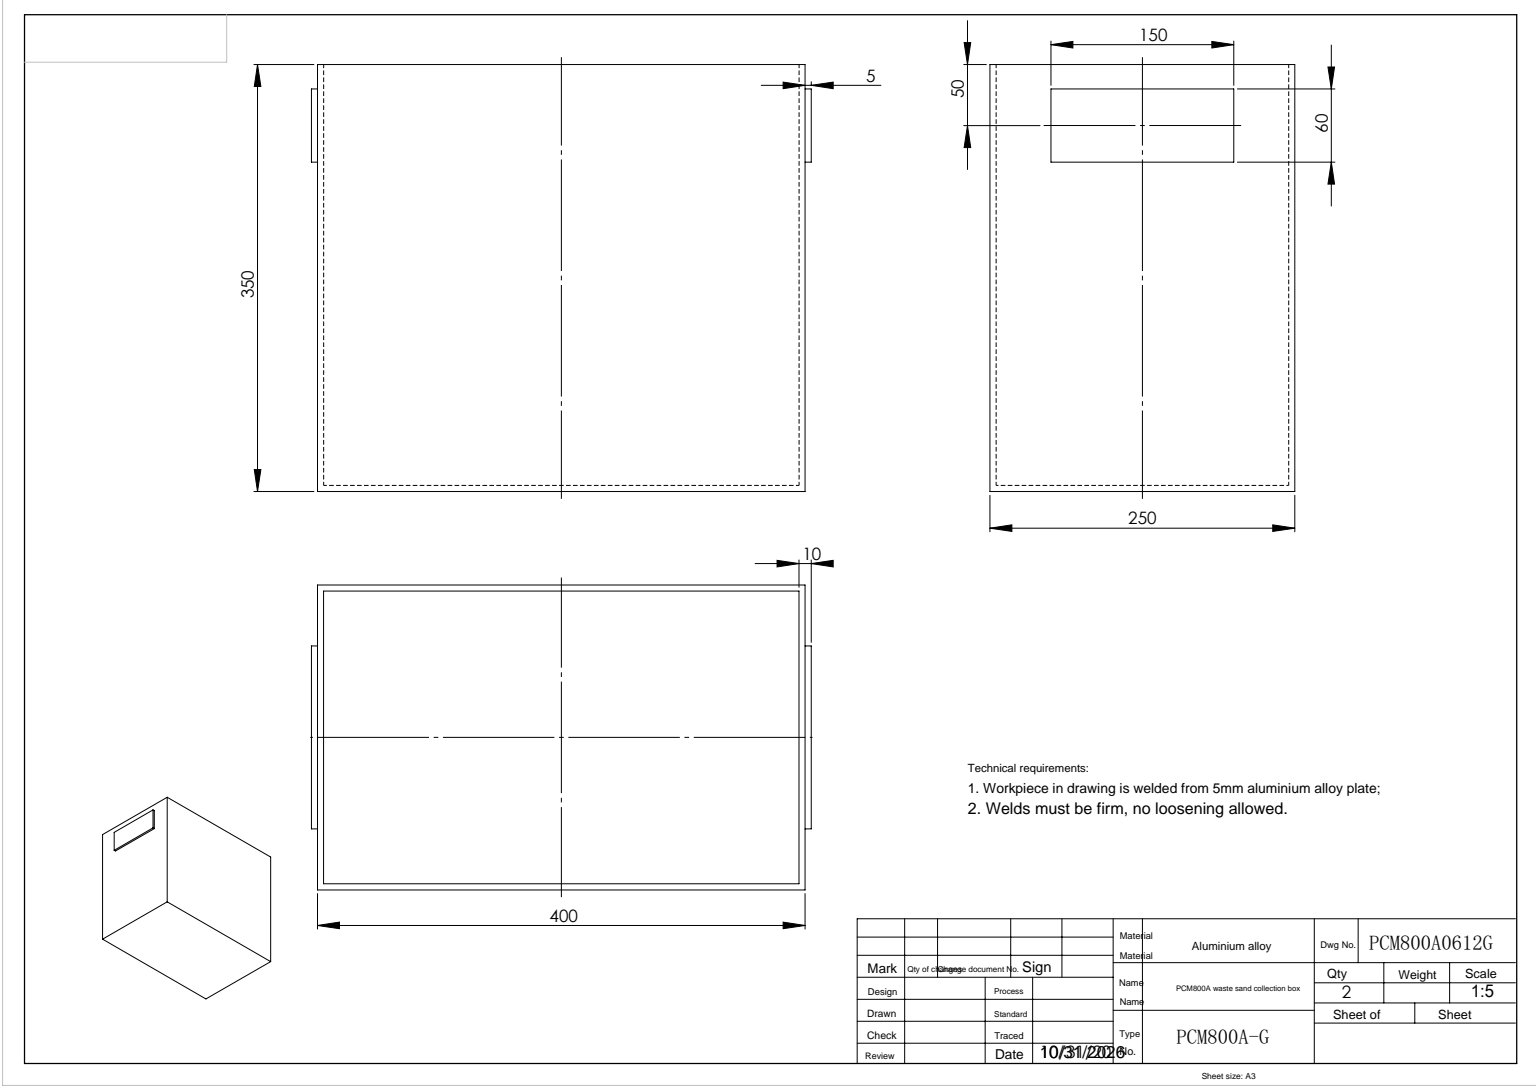
from build123d import *

# Parameters (mm, degrees)
SKETCH_1_W      = 400
SKETCH_1_H      = 250
EXTRUDE_1_DEPTH = 350
SHELL_1_T       = -5
SKETCH_2_W      = 150
SKETCH_2_H      = 60
EXTRUDE_2_DEPTH = 5
SKETCH_3_W      = 150
SKETCH_3_H      = 60
EXTRUDE_3_DEPTH = 5


with BuildPart() as part:
    # 草图1 → 凸台-拉伸1 (new body)
    with BuildSketch(Plane(origin=(0, 0, 0), x_dir=(1, 0, 0), z_dir=(0, 1, 0))):
        with Locations((200, 125)):
            Rectangle(SKETCH_1_W, SKETCH_1_H)
    extrude(amount=EXTRUDE_1_DEPTH)

    # 抽壳1
    shell_1_openings = [part.faces().sort_by_distance(p)[0] for p in [
        (200, 350, -125),
    ]]
    offset(amount=SHELL_1_T, openings=shell_1_openings, kind=Kind.INTERSECTION)

    # 草图2 → 凸台-拉伸2 (add)
    with BuildSketch(Plane(origin=(400, 0, 0), x_dir=(0, 0, -1), z_dir=(1, 0, 0))):
        with Locations((125, 300)):
            Rectangle(SKETCH_2_W, SKETCH_2_H)
    extrude(amount=EXTRUDE_2_DEPTH)

    # 草图3 → 凸台-拉伸3 (add)
    with BuildSketch(Plane.ZY):
        with Locations((-125, 300)):
            Rectangle(SKETCH_3_W, SKETCH_3_H)
    extrude(amount=EXTRUDE_3_DEPTH)


solid = part.part
